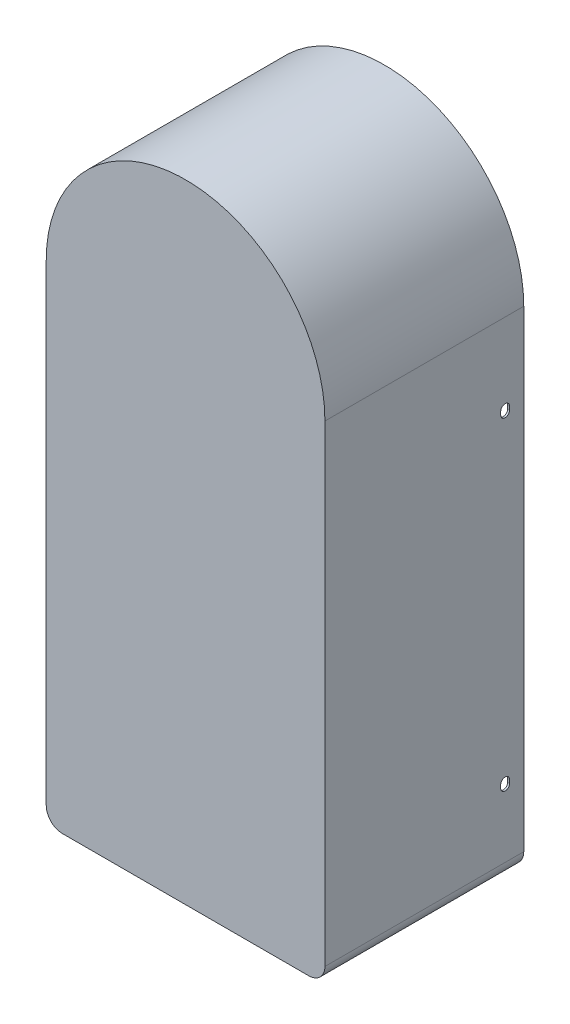
from build123d import *

# Parameters (mm, degrees)
BOSS_EXTRUDE1_DEPTH = 123
BOSS_EXTRUDE2_START = -1.2
BOSS_EXTRUDE2_DEPTH = 1.2
FILLET1_R           = 10
FILLET2_R           = 10
CUT_EXTRUDE1_DEPTH  = 318.612421042


with BuildPart() as part:
    # Sketch1 → Boss-Extrude1 (new body)
    with BuildSketch(Plane.XY):
        with BuildLine():
            Line((-86.2, -151.7), (-86.2, 150.5))
            ThreePointArc((-86.2, 150.5), (0, 236.7), (86.2, 150.5))
            Line((86.2, 150.5), (86.2, -151.7))
            Line((86.2, -151.7), (-86.2, -151.7))
        make_face()
        with BuildLine():
            Line((75, -150.5), (-75, -150.5))
            ThreePointArc((-75, -150.5), (-82.071067812, -147.571067812), (-85, -140.5))
            Line((-85, -140.5), (-85, 150.5))
            ThreePointArc((-85, 150.5), (0, 235.5), (85, 150.5))
            Line((85, 150.5), (85, -140.5))
            ThreePointArc((85, -140.5), (82.071067812, -147.571067812), (75, -150.5))
        make_face(mode=Mode.SUBTRACT)
    extrude(amount=BOSS_EXTRUDE1_DEPTH)

    # Sketch2 → Boss-Extrude2 (add)
    with BuildSketch(Plane.XY.offset(123).offset(BOSS_EXTRUDE2_START)):
        with BuildLine():
            Line((-86.2, 150.5), (-86.2, -151.7))
            Line((-86.2, -151.7), (86.2, -151.7))
            Line((86.2, -151.7), (86.2, 150.5))
            ThreePointArc((86.2, 150.5), (0, 236.7), (-86.2, 150.5))
        make_face()
    extrude(amount=BOSS_EXTRUDE2_DEPTH)

    # Fillet1
    fillet1_edges = [part.edges().sort_by_distance(p)[0] for p in [
        (-86.2, -151.7, 61.5),
    ]]
    fillet(fillet1_edges, radius=FILLET1_R)

    # Fillet2
    fillet2_edges = [part.edges().sort_by_distance(p)[0] for p in [
        (86.2, -151.7, 61.5),
    ]]
    fillet(fillet2_edges, radius=FILLET2_R)

    # Sketch3 → Cut-Extrude1 (cut, through all)
    with BuildSketch(Plane.ZY.offset(86.2)):
        with BuildLine():
            Line((8.75, 99.3), (8.75, 101.3))
            ThreePointArc((8.75, 101.3), (11.5, 104.05), (14.25, 101.3))
            Line((14.25, 101.3), (14.25, 99.3))
            ThreePointArc((14.25, 99.3), (11.5, 96.55), (8.75, 99.3))
        make_face()
        with BuildLine():
            Line((8.75, -100.7), (8.75, -98.7))
            ThreePointArc((8.75, -98.7), (11.5, -95.95), (14.25, -98.7))
            Line((14.25, -98.7), (14.25, -100.7))
            ThreePointArc((14.25, -100.7), (11.5, -103.45), (8.75, -100.7))
        make_face()
    extrude(amount=-CUT_EXTRUDE1_DEPTH, mode=Mode.SUBTRACT)


solid = part.part
